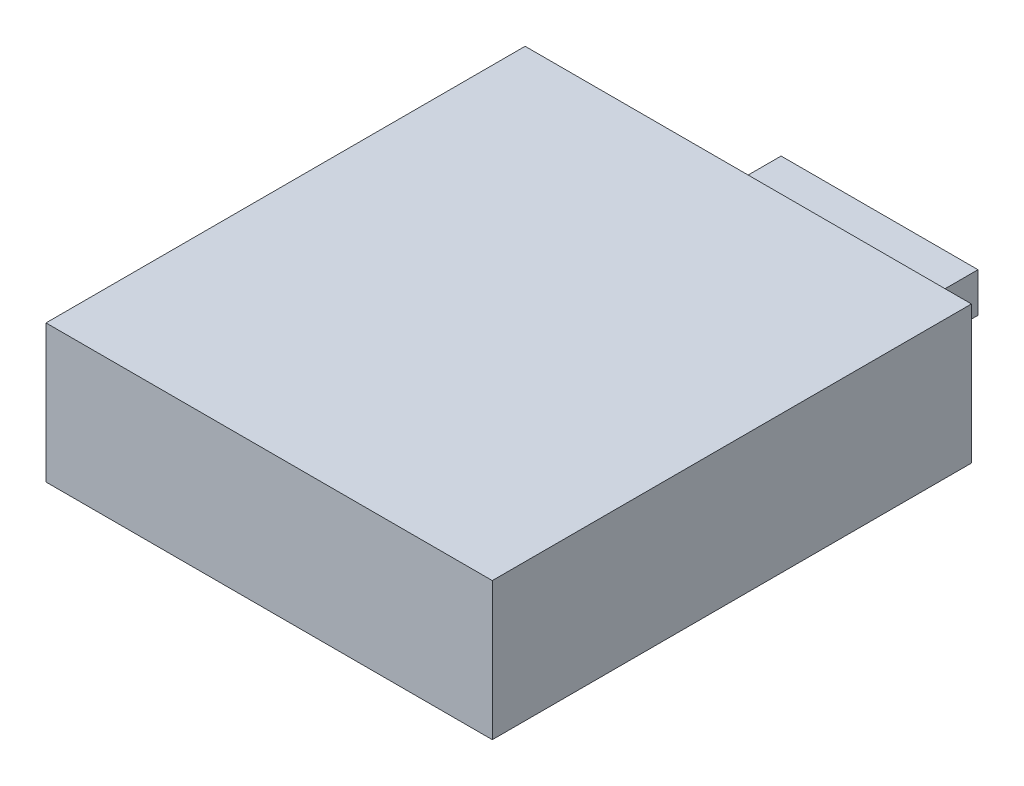
SolidWorks part; units mm, degrees
ref_plane "Front Plane" through (0, 0, 0) normal (0, 0, 1) x (1, 0, 0)
ref_plane "Top Plane" through (0, 0, 0) normal (0, 1, 0) x (1, 0, 0)
ref_plane "Right Plane" through (0, 0, 0) normal (1, 0, 0) x (0, 0, -1)
sketch "Sketch1" plane through (0, 0, 0) normal (0, 1, 0) x (1, 0, 0)
  line L1 (-34, -36.5) -> (34, -36.5)
  line L2 (-34, -36.5) -> (-34, 36.5)
  line L3 (-34, 36.5) -> (34, 36.5)
  line L4 (34, -36.5) -> (34, 36.5)
  line L5 (-34, -36.5) -> (34, 36.5) construction
  line L6 (-34, 36.5) -> (34, -36.5) construction
  point P0 (0, 0)
  dimension "D1" = 68
  dimension "D2" = 73
extrude "Boss-Extrude1" add sketch "Sketch1" along normal blind 21
sketch "Sketch2" plane through (0, 0, -36.5) normal (0, 0, -1) x (-1, 0, 0)
  line L0 (-34, 0) -> (34, 0) construction
  line L2 (-15, 0) -> (-15, 6.0202)
  line L3 (-15, 6.0202) -> (15, 6.0202)
  line L4 (15, 0) -> (15, 6.0202)
  line L5 (0, 0) -> (15, 6.0202) construction
  line L6 (-15, 6.0202) -> (0, 0) construction
  line L7 (-15, 0) -> (15, 0)
  point P0 (0, 0)
  dimension "D1" = 30
extrude "Boss-Extrude2" add sketch "Sketch2" along normal blind 20
sketch "Sketch3" plane through (0, 6.0202, 0) normal (0, 1, 0) x (1, 0, 0)
  line L0 (15, 56.5) -> (15, 36.5) construction
  circle A0 centre (9.5, 48.2568) radius 3
  circle A1 centre (-9.5, 48.2568) radius 3
  dimension "D1" = 19
  dimension "D2" = 6
  dimension "D3" = 6
  dimension "D4" = 5.5
extrude "Cut-Extrude1" cut sketch "Sketch3" against normal blind 20
